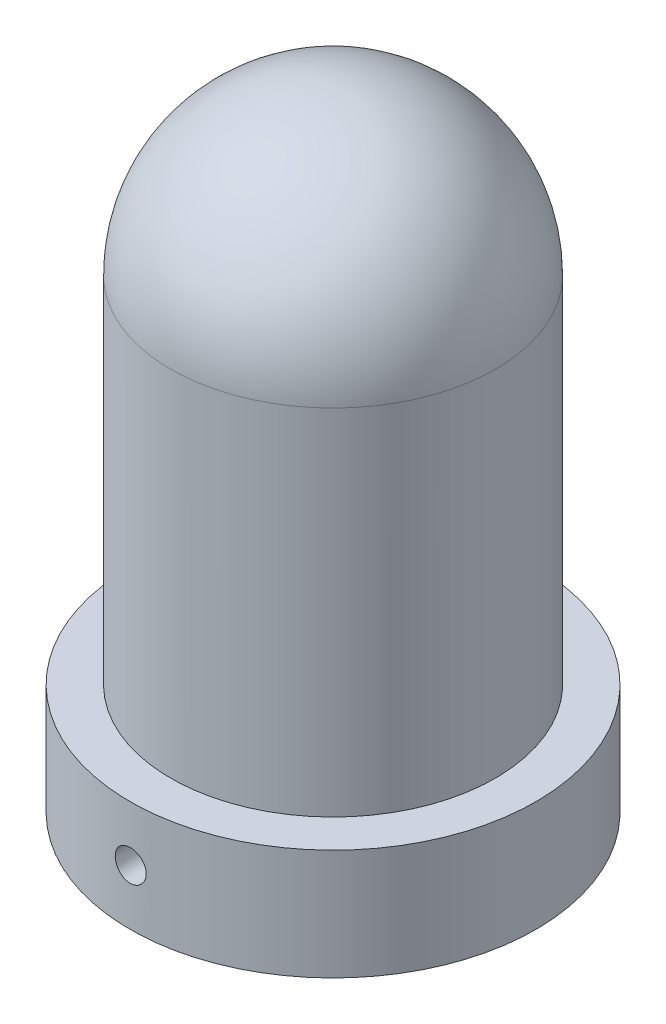
from build123d import *

# Parameters (mm, degrees)
M5_TAPPED_HOLE1_D     = 4.2
M5_TAPPED_HOLE1_DEPTH = 30
M5_TAPPED_HOLE1_TIP   = 1.2618073
CHAMFER1_SIZE         = 2


with BuildPart() as part:
    # Sketch1 → Revolve2 (revolve)
    with BuildSketch(Plane.XY, mode=Mode.PRIVATE) as revolve2_sk:
        with BuildLine():
            Line((-22, 63), (-22, 15))
            Line((-22, 15), (-27.5, 15))
            Line((-27.5, 15), (-27.5, 0))
            Line((-27.5, 0), (-17.5, 0))
            Line((-17.5, 0), (-17.5, 20))
            Line((-17.5, 20), (-17, 20))
            Line((-17, 20), (-17, 63))
            ThreePointArc((-17, 63), (-12.02081528, 75.02081528), (0, 80))
            Line((0, 80), (0, 85))
            ThreePointArc((0, 85), (-15.556349186, 78.556349186), (-22, 63))
        make_face()
    revolve(revolve2_sk.sketch.rotate(Axis((0, 0, 0), (0, 1, 0)), 270), axis=Axis((0, 0, 0), (0, 1, 0)))

    # M5 Tapped Hole1
    with Locations(Plane(origin=(-0.002180136, 7.524181673, 27.499999914), x_dir=(0.999999996858, 0, 7.9277686e-05), z_dir=(-7.9277686e-05, 0, 0.999999996858))):
        with Locations((0, 0)):
            Hole(M5_TAPPED_HOLE1_D / 2, depth=M5_TAPPED_HOLE1_DEPTH)
            with Locations((0, 0, -(M5_TAPPED_HOLE1_DEPTH + M5_TAPPED_HOLE1_TIP / 2))):  # 118° drill point
                Cone(0, M5_TAPPED_HOLE1_D / 2, M5_TAPPED_HOLE1_TIP, mode=Mode.SUBTRACT)

    # Chamfer1
    chamfer1_edges = [part.edges().sort_by_distance(p)[0] for p in [
        (0, 0, 17.5),
    ]]
    chamfer(chamfer1_edges, length=CHAMFER1_SIZE)


solid = part.part
